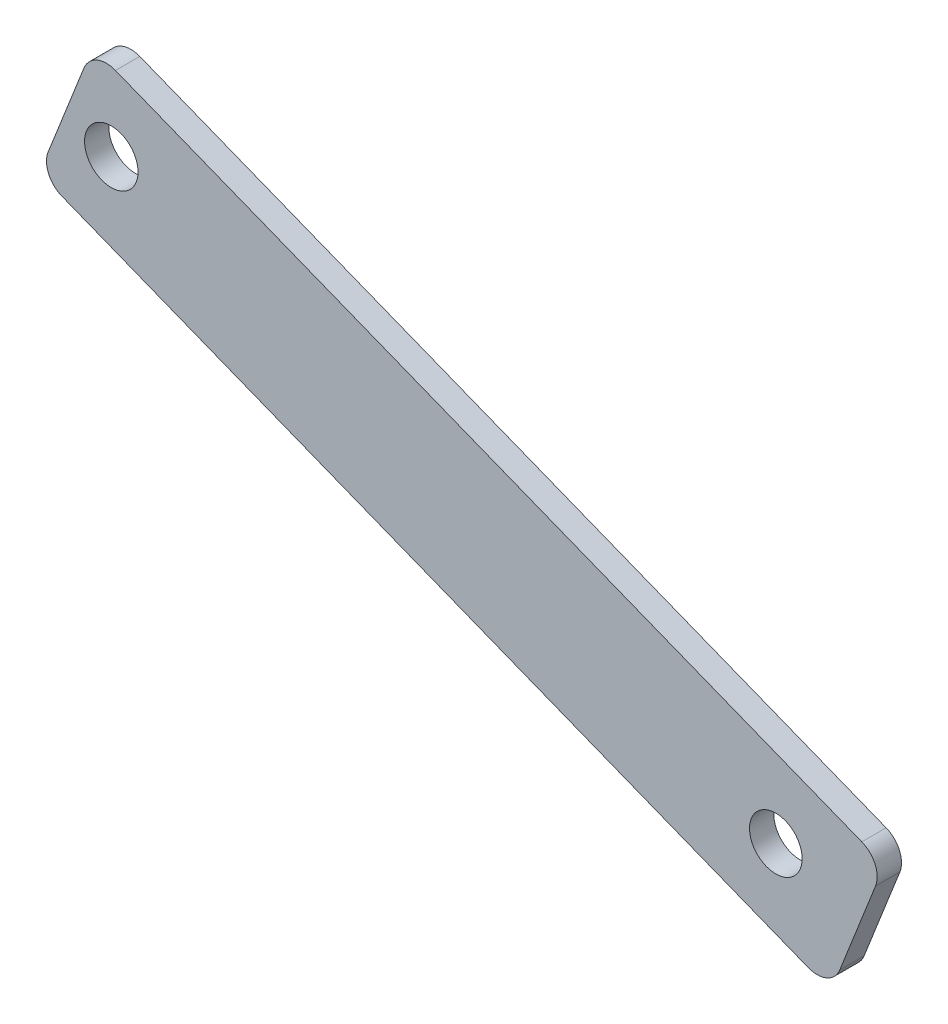
SolidWorks part; units mm, degrees
material "Q235铸造"
ref_plane "前视基准面" through (0, 0, 0) normal (0, 0, 1) x (1, 0, 0)
ref_plane "上视基准面" through (0, 0, 0) normal (0, 1, 0) x (1, 0, 0)
ref_plane "右视基准面" through (0, 0, 0) normal (1, 0, 0) x (0, 0, -1)
ref_plane "基准面1" through (0, 0, -1083.2374) normal (0, 0, 1) x (1, 0, 0)
sketch "草图1" plane through (0, 0, -1083.2374) normal (0, 0, 1) x (1, 0, 0)
  line L0 (-135.5157, 493.6263) -> (171.4013, 372.3748)
  line L1 (-148.4905, 488.0001) -> (-163.1877, 450.7981)
  line L2 (177.0275, 359.4) -> (162.3304, 322.1979)
  line L3 (-157.5615, 437.8232) -> (149.3556, 316.5717)
  line L4 (17.9428, 433.0006) -> (48.403, 510.1028) construction
  line L5 (-137.2381, 462.0505) -> (262.4652, 304.1426) construction
  arc A0 (171.4013, 372.3748) -> (177.0275, 359.4) centre (167.727, 363.0743) cw
  arc A1 (162.3304, 322.1979) -> (149.3556, 316.5717) centre (153.0298, 325.8722) cw
  arc A2 (-163.1877, 450.7981) -> (-157.5615, 437.8232) centre (-153.8872, 447.1238) ccw
  arc A3 (-148.4905, 488.0001) -> (-135.5157, 493.6263) centre (-139.19, 484.3258) cw
  circle A4 centre (-137.2381, 462.0505) radius 11
  circle A5 centre (136.039, 354.0889) radius 10.8245
  dimension "D1" = 10
  dimension "D5" = 22
  dimension "D6" = 293.83
  dimension "D2" = 60
  dimension "D3" = 350
  dimension "D4" = 20
extrude "凸台-拉伸1" add sketch "草图1" along normal blind 10 from offset 40
